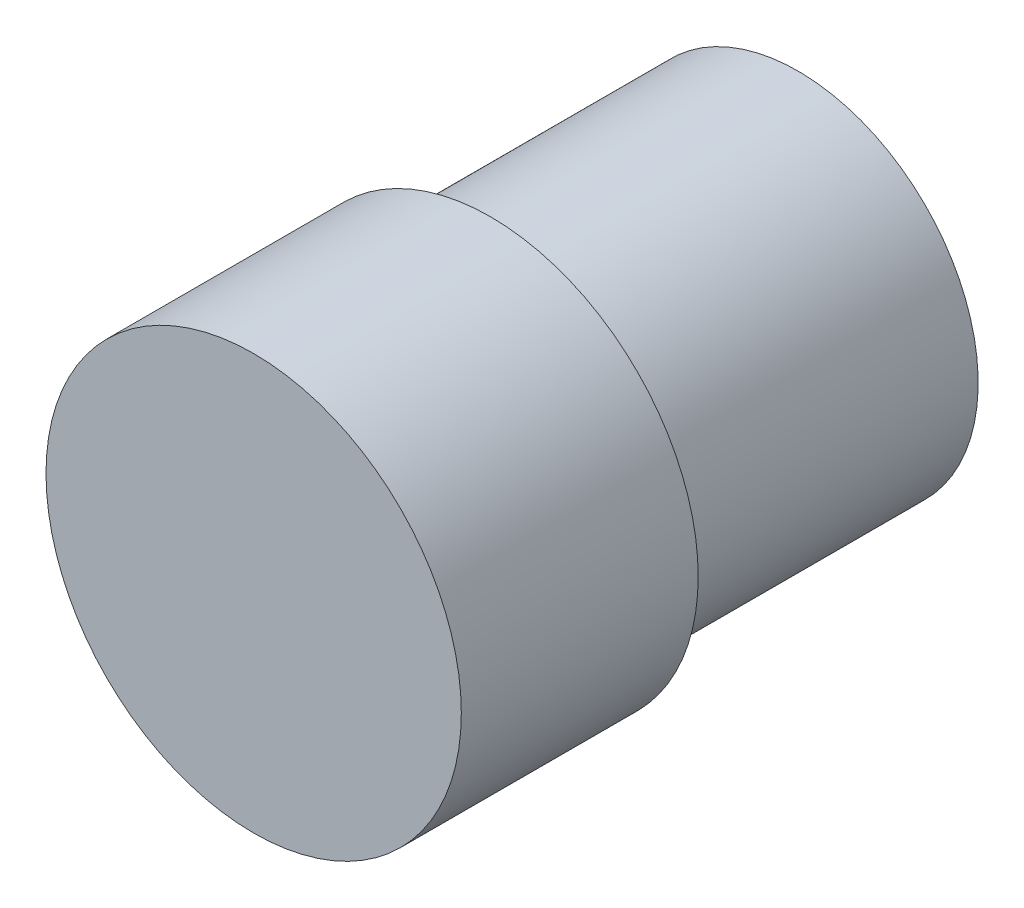
SolidWorks part; units mm, degrees
ref_plane "Front Plane" through (0, 0, 0) normal (0, 0, 1) x (1, 0, 0)
ref_plane "Top Plane" through (0, 0, 0) normal (0, 1, 0) x (1, 0, 0)
ref_plane "Right Plane" through (0, 0, 0) normal (1, 0, 0) x (0, 0, -1)
sketch "Sketch1" plane through (0, 0, 0) normal (0, 0, 1) x (1, 0, 0)
  circle A0 centre (50.5319, -8.1057) radius 6.75
extrude "Boss-Extrude1" add sketch "Sketch1" along normal blind 4.5
sketch "Sketch2" plane through (0, 0, 0) normal (0, 0, -1) x (-1, 0, 0)
  circle A0 centre (-50.5319, -8.1057) radius 6.75
  dimension "D1" = 13.5
extrude "Boss-Extrude2" add sketch "Sketch2" along normal blind 3.2
sketch "Sketch3" plane through (0, 0, -3.2) normal (0, 0, -1) x (-1, 0, 0)
  circle A0 centre (-50.5319, -8.1057) radius 5.85
extrude "Boss-Extrude3" add sketch "Sketch3" along normal blind 10
